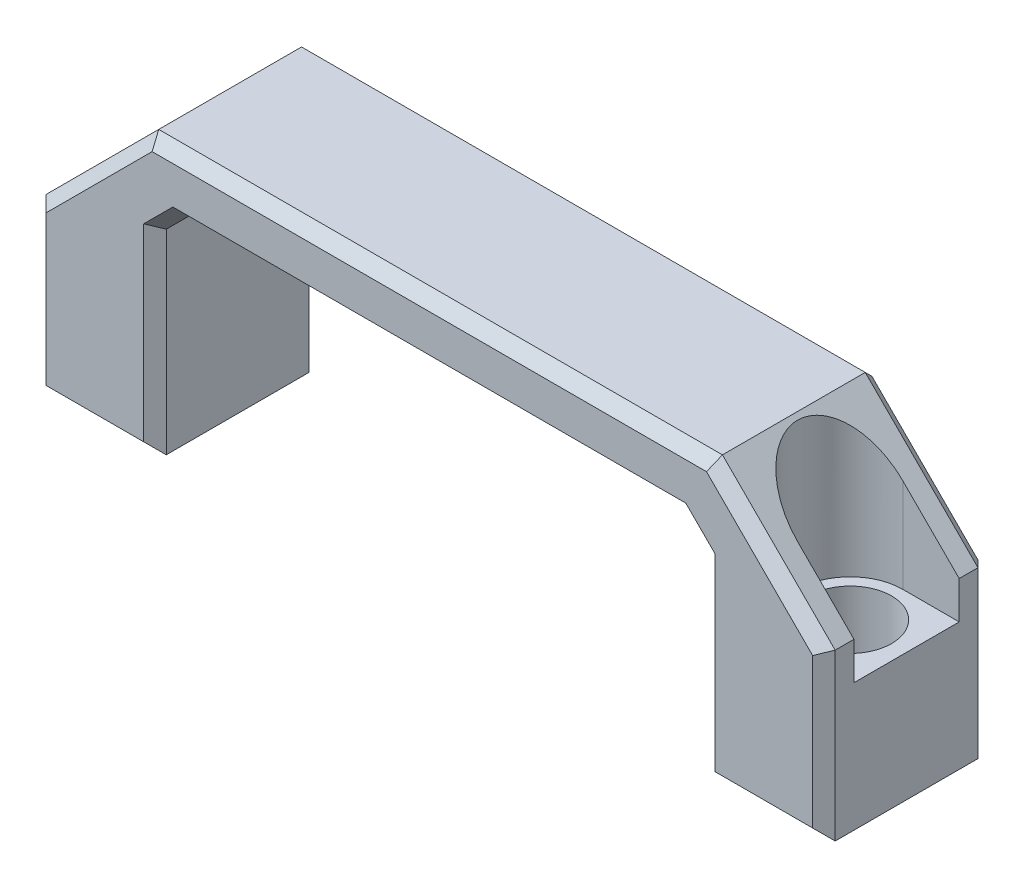
from build123d import *

# Parameters (mm, degrees)
EXTRUDE_1_DEPTH              = 11
HOLE_WIZARD_M6_1_D           = 6.5
HOLE_WIZARD_M6_1_CBORE_D     = 11
HOLE_WIZARD_M6_1_CBORE_DEPTH = 30
CUT_EXTRUDE_1_DEPTH          = 20
CHAMFER_1_SIZE               = 1.5


with BuildPart() as part:
    # 草图1 → 凸台-拉伸1 (new, symmetric)
    with BuildSketch(Plane.XY):
        Polygon((-52.5, 0), (-36.5, 0), (-36.5, 26), (-33.5, 29), (33.5, 29), (36.5, 26), (36.5, 0), (52.5, 0), (52.5, 22), (37.5, 37), (-37.5, 37), (-52.5, 22), align=None)
    extrude(amount=EXTRUDE_1_DEPTH, both=True)

    # M6 六角凹头螺钉的柱形沉头孔1 (through all)
    with Locations(Plane(origin=(0, 37, 0), x_dir=(1, 0, 0), z_dir=(0, 1, 0))):
        with Locations((-45, 0), (45, 0)):
            CounterBoreHole(HOLE_WIZARD_M6_1_D / 2, HOLE_WIZARD_M6_1_CBORE_D / 2, HOLE_WIZARD_M6_1_CBORE_DEPTH)

    # 草图4 → 切除-拉伸1 (cut)
    with BuildSketch(Plane(origin=(0, 37, 0), x_dir=(1, 0, 0), z_dir=(0, 1, 0))):
        with BuildLine():
            Line((-52.5, 7), (-45, 7))
            ThreePointArc((-45, 7), (-38, 0), (-45, -7))
            Line((-45, -7), (-52.5, -7))
            ThreePointArc((-52.5, -7), (-59.5, 0), (-52.5, 7))
        make_face()
        with BuildLine():
            Line((52.5, 7), (45, 7))
            ThreePointArc((45, 7), (38, 0), (45, -7))
            Line((45, -7), (52.5, -7))
            ThreePointArc((52.5, -7), (59.5, 0), (52.5, 7))
        make_face()
    extrude(amount=-CUT_EXTRUDE_1_DEPTH, mode=Mode.SUBTRACT)

    # 倒角1
    chamfer_1_edges = [part.edges().sort_by_distance(p)[0] for p in [
        (-36.5, 13, 11),
        (-45, 29.5, -11),
        (0, 37, -11),
        (45, 29.5, -11),
        (52.5, 11, -11),
        (44.5, 0, -11),
        (36.5, 13, -11),
        (-35, 27.5, 11),
        (35, 27.5, -11),
        (0, 29, -11),
        (-35, 27.5, -11),
        (-36.5, 13, -11),
        (-44.5, 0, -11),
        (-52.5, 11, -11),
        (0, 29, 11),
        (35, 27.5, 11),
        (36.5, 13, 11),
        (44.5, 0, 11),
        (52.5, 11, 11),
        (45, 29.5, 11),
        (0, 37, 11),
        (-45, 29.5, 11),
        (-52.5, 11, 11),
        (-44.5, 0, 11),
    ]]
    chamfer(chamfer_1_edges, length=CHAMFER_1_SIZE)


solid = part.part
